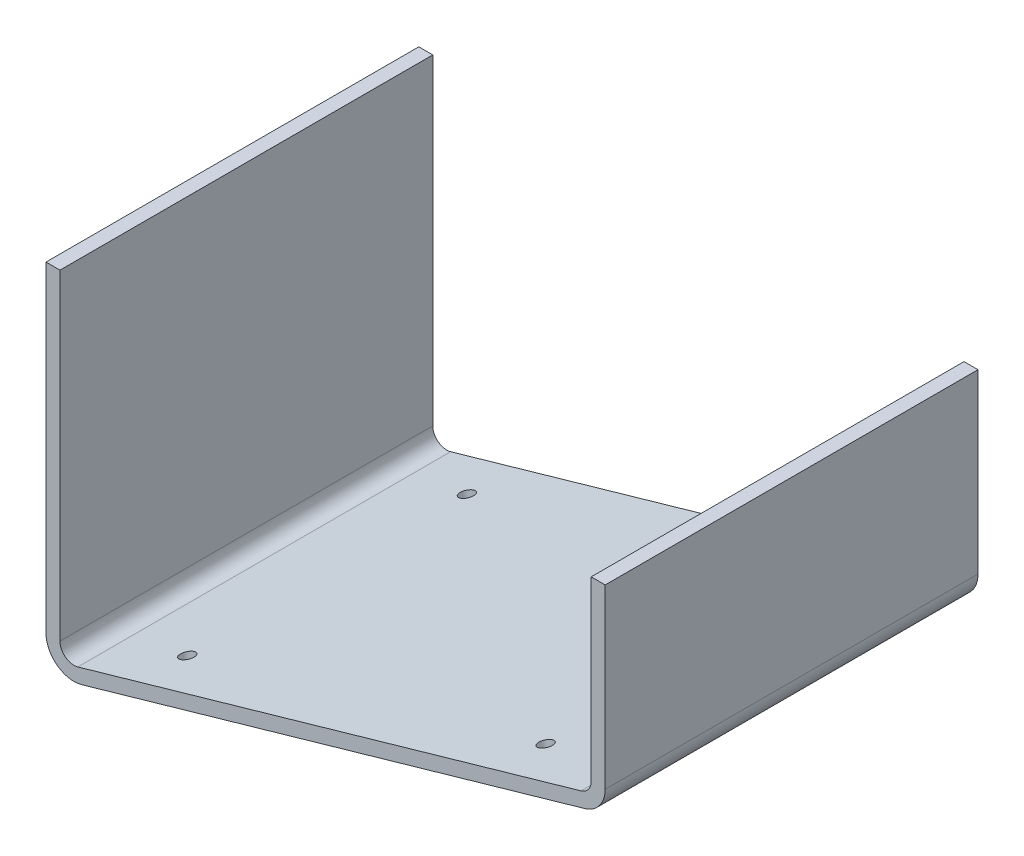
from build123d import *

# Parameters (mm, degrees)
BOSS_EXTRUDE1_DEPTH = 160
SKETCH2_R           = 3
CUT_EXTRUDE1_DEPTH  = 8


with BuildPart() as part:
    # Sketch1 → Boss-Extrude1 (new body)
    with BuildSketch(Plane.XY):
        with BuildLine():
            Line((0, 0), (0, -137.894354723))
            ThreePointArc((0, -137.894354723), (4.778219722, -147.477980843), (15.30764827, -149.429495074))
            Line((15.30764827, -149.429495074), (231.30764827, -87.49249175))
            ThreePointArc((231.30764827, -87.49249175), (237.583626121, -83.179131677), (240, -75.957351399))
            Line((240, -75.957351399), (240, 0))
            Line((240, 0), (234, 0))
            Line((234, 0), (234, -75.957351399))
            ThreePointArc((234, -75.957351399), (232.79181306, -79.568241538), (229.653824135, -81.724921574))
            Line((229.653824135, -81.724921574), (13.653824135, -143.661924898))
            ThreePointArc((13.653824135, -143.661924898), (8.389109861, -142.686167783), (6, -137.894354723))
            Line((6, -137.894354723), (6, 0))
            Line((6, 0), (0, 0))
        make_face()
    extrude(amount=BOSS_EXTRUDE1_DEPTH)

    # Sketch2 → Cut-Extrude1 (cut)
    with BuildSketch(Plane(origin=(40.755797191, -142.132355795, 0), x_dir=(0.9612616959383188, 0.2756373558169997, 0), z_dir=(0.27563735581699966, -0.9612616959383187, 0))):
        with Locations((1.601767174, 140)):
            Circle(SKETCH2_R)
        with Locations((1.601767174, 20)):
            Circle(SKETCH2_R)
        with Locations((161.601767174, 140)):
            Circle(SKETCH2_R)
        with Locations((161.601767174, 20)):
            Circle(SKETCH2_R)
    extrude(amount=-CUT_EXTRUDE1_DEPTH, mode=Mode.SUBTRACT)


solid = part.part
